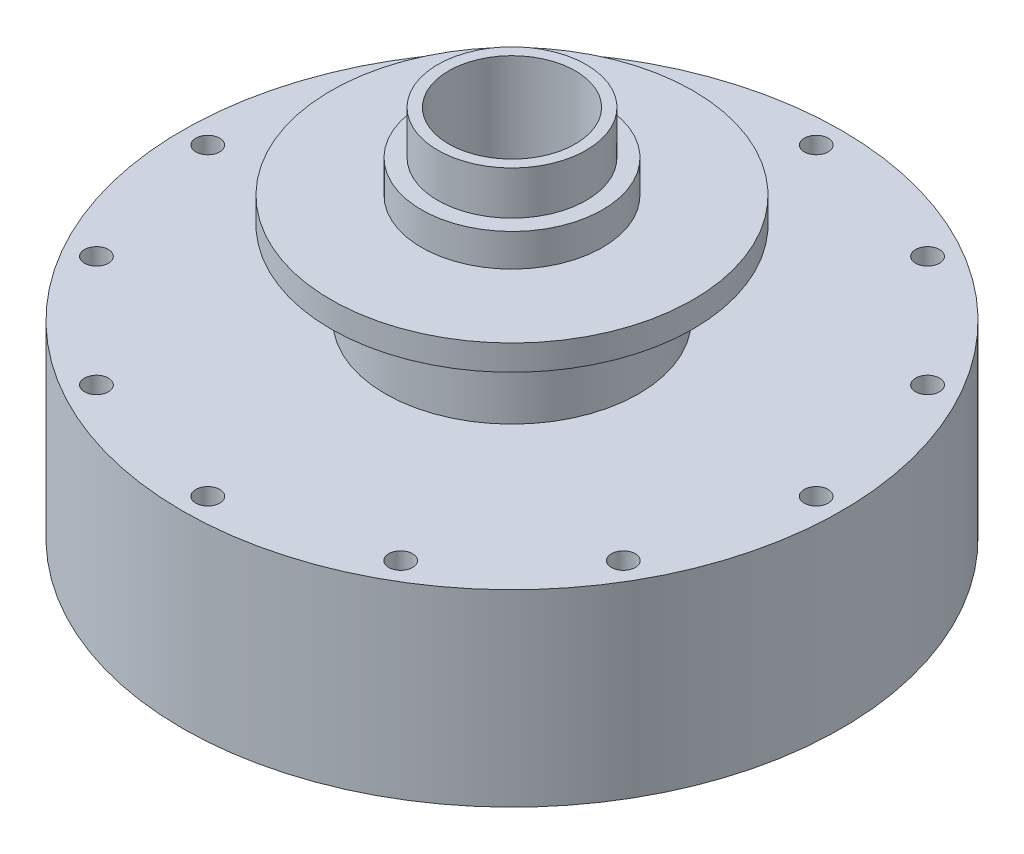
SolidWorks part; units mm, degrees
material "标准件"
ref_plane "前视基准面" through (0, 0, 0) normal (0, 0, 1) x (1, 0, 0)
ref_plane "上视基准面" through (0, 0, 0) normal (0, 1, 0) x (1, 0, 0)
ref_plane "右视基准面" through (0, 0, 0) normal (1, 0, 0) x (0, 0, -1)
sketch "草图1" plane through (0, 0, 0) normal (0, 0, 1) x (1, 0, 0)
  line L0 (0, 0) -> (0, 109) construction
  line L1 (0, 0) -> (70, 0)
  line L2 (70, 0) -> (70, 6)
  line L3 (70, 6) -> (91, 6)
  line L4 (91, 6) -> (91, 58)
  line L5 (91, 58) -> (50, 58)
  line L6 (50, 58) -> (50, 88)
  line L7 (50, 88) -> (25, 88)
  line L8 (25, 88) -> (25, 97)
  line L9 (25, 97) -> (20.5, 97)
  line L10 (20.5, 97) -> (20.5, 109)
  line L11 (20.5, 109) -> (0, 109)
  line L12 (0, 0) -> (0, 109)
  dimension "D1" = 182
  dimension "D2" = 58
  dimension "D3" = 100
  dimension "D4" = 50
  dimension "D5" = 41
  dimension "D6" = 6
  dimension "D7" = 70
  dimension "D8" = 97
  dimension "D9" = 88
  dimension "D10" = 109
revolve "旋转1" add sketch "草图1" angle 360 about L0
sketch "草图2" plane through (0, 109, 0) normal (0, 1, 0) x (1, 0, 0)
  circle A0 centre (0, 0) radius 17.5
  dimension "D1" = 35
extrude "切除-拉伸1" cut sketch "草图2" against normal through all
hole_wizard "M6 间隙孔1" positions "草图3" profile "草图4" hole size "M6" standard "ISO" end condition through all
sketch "草图3" plane through (0, 58, 0) normal (0, 1, 0) x (1, 0, 0)
  line L0 (0, 0) -> (0, 91) construction
  line L2 (0, 0) -> (0, 84) construction
  circle A0 centre (0, 0) radius 91 construction
  point P0 (0, 84)
  point P14 (42, 72.7461)
  point P15 (72.7461, 42)
  point P16 (84, 0)
  point P17 (72.7461, -42)
  point P18 (42, -72.7461)
  point P19 (0, -84)
  point P20 (-42, -72.7461)
  point P23 (-72.7461, -42)
  point P24 (-84, 0)
  point P25 (-72.7461, 42)
  point P26 (-42, 72.7461)
  dimension "D3" = 84
  dimension "D2" = 12
sketch "草图4" plane through (0, 58, -84) normal (1, 0, 0) x (0, 0, 1)
  line L0 (0, 0) -> (0, 58)
  line L1 (0, 58) -> (3.3, 58)
  line L2 (3.3, 58) -> (3.3, 0)
  line L5 (3.3, 0) -> (0, 0)
  line L11 (0, -6.35) -> (0, 107.95) construction
  dimension "通孔孔直径" = 6.6
  dimension "通孔孔深度" = 58
ref_plane "基准面1" through (0, 84.5, 0) normal (0, 1, 0) x (1, 0, 0)
sketch "草图6" plane through (0, 84.5, 0) normal (0, 1, 0) x (1, 0, 0)
  circle A0 centre (0, 0) radius 48.75
  dimension "D1" = 97.5
hole_wizard "M8 螺纹孔1" positions "草图7" profile "草图8" tap size "M8" standard "ISO"
sketch "草图7" plane through (0, 0, 0) normal (0, -1, 0) x (-1, 0, 0)
  line L0 (0, 0) -> (0, 58) construction
  line L1 (0, 0) -> (0, 58) construction
  point P0 (0, 58)
  point P10 (41.0122, 41.0122)
  point P11 (58, 0)
  point P12 (41.0122, -41.0122)
  point P13 (0, -58)
  point P14 (-41.0122, -41.0122)
  point P15 (-58, 0)
  point P16 (-41.0122, 41.0122)
  dimension "D3" = 58
  dimension "D2" = 8
sketch "草图8" plane through (0, 0, -58) normal (1, 0, 0) x (0, 0, -1)
  line L0 (0, 0) -> (0, 21.7929)
  line L1 (0, 21.7929) -> (3.4, 19.75)
  line L2 (3.4, 19.75) -> (3.4, 0)
  line L5 (3.4, 0) -> (0, 0)
  line L10 (0, 21.7929) -> (-3.4, 19.75) construction
  line L11 (0, -6.35) -> (0, 107.95) construction
  dimension "螺纹孔钻头直径" = 6.8
  dimension "螺纹孔钻头深度" = 19.75
  dimension "导头角度" = 118
sketch "草图9" plane through (0, 0, 0) normal (0, 0, 1) x (1, 0, 0)
  line L0 (50, 58) -> (50, 88) construction
  line L1 (50, 81) -> (35, 81)
  line L2 (50, 81) -> (50, 58)
  line L3 (50, 58) -> (35, 58)
  line L4 (35, 81) -> (35, 58)
  line L5 (91, 58) -> (-91, 58) construction
  line L6 (50, 88) -> (-50, 88) construction
  dimension "D1" = 7
  dimension "D2" = 15
revolve "切除-旋转1" cut sketch "草图9" angle 360 about axis through (0, 0, 0) along (0, -1, 0)
